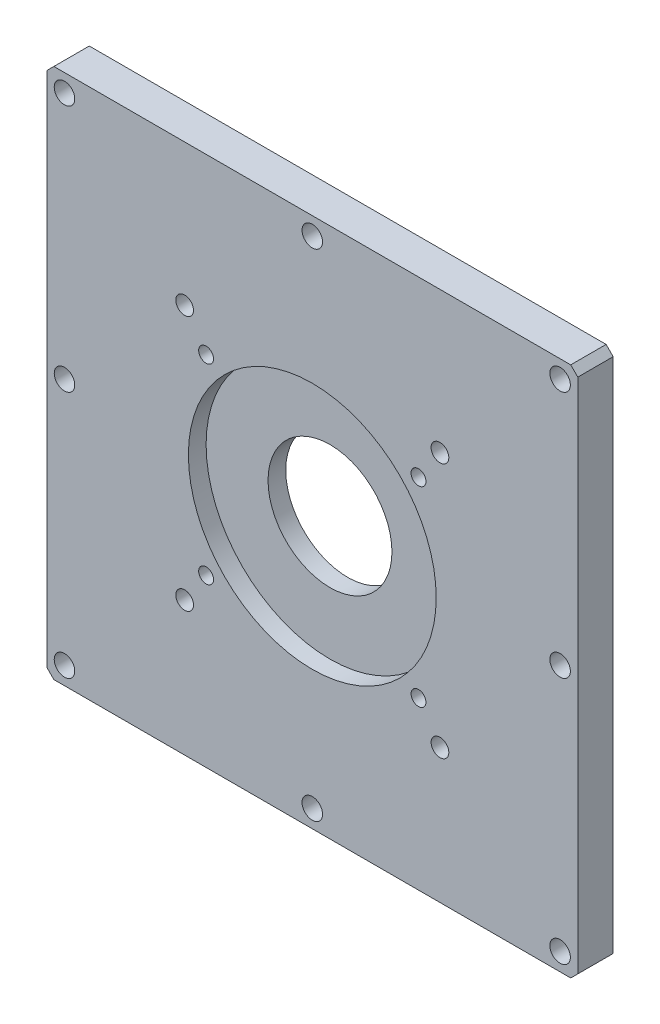
SolidWorks part; units mm, degrees
material "6061Al"
ref_plane "前视基准面" through (0, 0, 0) normal (0, 0, 1) x (1, 0, 0)
ref_plane "上视基准面" through (0, 0, 0) normal (0, 1, 0) x (1, 0, 0)
ref_plane "右视基准面" through (0, 0, 0) normal (1, 0, 0) x (0, 0, -1)
sketch "草图1" plane through (0, 0, 0) normal (0, 0, 1) x (1, 0, 0)
  line L1 (-75, -75) -> (75, -75)
  line L2 (-75, -75) -> (-75, 75)
  line L3 (-75, 75) -> (75, 75)
  line L4 (75, -75) -> (75, 75)
  line L5 (-75, -75) -> (75, 75) construction
  line L6 (-75, 75) -> (75, -75) construction
  point P0 (0, 0)
  dimension "D1" = 150
  dimension "D2" = 150
extrude "凸台-拉伸1" add sketch "草图1" along normal mid plane 10
sketch "草图3" plane through (0, 0, -5) normal (0, 0, -1) x (-1, 0, 0)
  circle A0 centre (0, -1) radius 17.5
  point P2 (0, 0)
  point P3 (0, -1)
  dimension "D1" = 35
extrude "切除-拉伸1" cut sketch "草图3" against normal through all
hole_wizard "M5 间隙孔1" positions "草图4" profile "草图5" hole size "M5" standard "ISO" end condition through all
sketch "草图4" plane through (0, 0, -5) normal (0, 0, -1) x (-1, 0, 0)
  point P0 (-70, 70)
  point P3 (-70, 0)
  point P6 (-70, -70)
  point P9 (0, -70)
  point P12 (70, -70)
  point P15 (70, 0)
  point P18 (70, 70)
  point P21 (0, 70)
sketch "草图5" plane through (70, 70, -5) normal (1, 0, 0) x (0, 1, 0)
  line L0 (0, 0) -> (0, 10)
  line L1 (0, 10) -> (2.9, 10)
  line L2 (2.9, 10) -> (2.9, 0)
  line L5 (2.9, 0) -> (0, 0)
  line L11 (0, -6.35) -> (0, 107.95) construction
  dimension "通孔孔直径" = 5.8
  dimension "通孔孔深度" = 10
chamfer "倒角1" distance 2 angle 45 4 edges at (-75, -75, 0) (75, -75, 0) (75, 75, 0) (-75, 75, 0)
sketch "草图6" plane through (0, 0, 5) normal (0, 0, 1) x (1, 0, 0)
  circle A0 centre (0, -1) radius 35
  dimension "D1" = 70
extrude "切除-拉伸2" cut sketch "草图6" against normal blind 5
hole_wizard "M6 螺纹孔1" positions "草图7" profile "草图8" tap size "M6" standard "GB" end condition up to next
sketch "草图7" plane through (0, 0, 5) normal (0, 0, 1) x (1, 0, 0)
  line L1 (36.06, -37.06) -> (-36.06, -37.06)
  line L2 (36.06, -37.06) -> (36.06, 35.06)
  line L3 (36.06, 35.06) -> (-36.06, 35.06)
  line L4 (-36.06, -37.06) -> (-36.06, 35.06)
  line L5 (36.06, -37.06) -> (-36.06, 35.06) construction
  line L6 (36.06, 35.06) -> (-36.06, -37.06) construction
  point P0 (-36.06, 35.06)
  point P3 (0, -1)
  point P7 (36.06, -37.06)
  point P8 (36.06, 35.06)
  point P9 (-36.06, -37.06)
  point P42 (0, 0)
  point P43 (-4.3241, -12.9425)
  point P44 (-36.9295, 30.3129)
  point P45 (-0.8695, -5.7471)
  point P46 (-1.211, -3.0298)
  point P47 (0, -1)
  dimension "D1" = 72.12
sketch "草图8" plane through (-36.06, 35.06, 5) normal (1, 0, 0) x (0, -1, 0)
  line L0 (0, 0) -> (0, 10)
  line L1 (0, 10) -> (2.5, 10)
  line L2 (2.5, 10) -> (2.5, 0)
  line L5 (2.5, 0) -> (0, 0)
  line L11 (0, -6.35) -> (0, 107.95) construction
  dimension "通孔螺纹孔钻头直径" = 5
  dimension "通孔螺纹孔钻头深度" = 10
cosmetic thread "孔螺蚊线1" parameters "D2"=6
cosmetic thread "孔螺蚊线2" parameters "D2"=6
cosmetic thread "孔螺蚊线3" parameters "D2"=6
cosmetic thread "孔螺蚊线4" parameters "D2"=6
hole_wizard "M5 螺纹孔1" positions "草图9" profile "草图10" tap size "M5" standard "GB" end condition through all
sketch "草图9" plane through (0, 0, -5) normal (0, 0, -1) x (-1, 0, 0)
  point P0 (-30, 26)
  point P3 (30, 26)
  point P6 (-30, -28)
  point P9 (30, -28)
sketch "草图10" plane through (30, 26, -5) normal (1, 0, 0) x (0, 1, 0)
  line L0 (0, 0) -> (0, 10)
  line L1 (0, 10) -> (2.1, 10)
  line L2 (2.1, 10) -> (2.1, 0)
  line L5 (2.1, 0) -> (0, 0)
  line L11 (0, -6.35) -> (0, 107.95) construction
  dimension "通孔螺纹孔钻头直径" = 4.2
  dimension "通孔螺纹孔钻头深度" = 10
cosmetic thread "孔螺蚊线5" parameters "D2"=5
cosmetic thread "孔螺蚊线6" parameters "D2"=5
cosmetic thread "孔螺蚊线7" parameters "D2"=5
cosmetic thread "孔螺蚊线8" parameters "D2"=5
